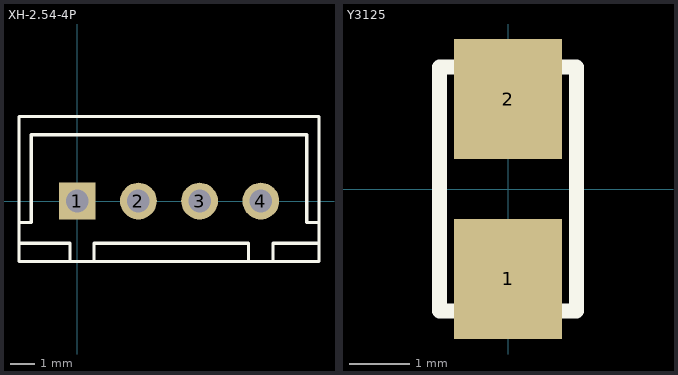
[diagram p0: the footprints below, top view; thin cyan lines are the x and y axes]
# Altium footprint library MISC82162-2.PcbLib: 66 footprints (part 5 of 5)
Each footprint in its own frame and in the unit in brackets; x right, y up, seen from the top. Pads: shape width x height; smd on the part's side, far side on the other; paste and mask are expansions set on the pad; w line width, h text height; cw(c..) or ccw(c..) is an arc to the next point about the centre after c.

## XH-2.54-4P [mil]
pads (4):
  rect 60x60 hole 37: 1(0,0)
  round 60 hole 37: 2(100,0) 3(200,0) 4(300,0)
Top Overlay:
  lines w5: -95,-68.9 -11.81,-68.9 -11.81,-98.43 ; -95,-35 -75,-35 -75,108.27 375,108.27 375,-35 395,-35 ; 27.56,-98.43 27.56,-68.9 280,-68.9 280,-98.43 ; 320,-98.43 320,-68.9 395,-68.9 ; -95,-98.43 -95,137.8 395,137.8 395,-98.43 -95,-98.43
Bottom Overlay:
  region: 264.17,-43.31 232.68,-43.31 232.68,55.12 264.17,55.12
  region: 165.75,-43.31 134.25,-43.31 134.25,55.12 165.75,55.12
  region: 67.32,-43.31 35.83,-43.31 35.83,55.12 67.32,55.12

## Y3125 [mm]
pads (2):
  rect 1.8x2 smd: 1(0,-1.5) 2(0,1.5)
Top Overlay:
  lines w0.254: -1.143,-2.032 1.143,-2.032 1.143,2.032 -1.143,2.032 -1.143,-2.032